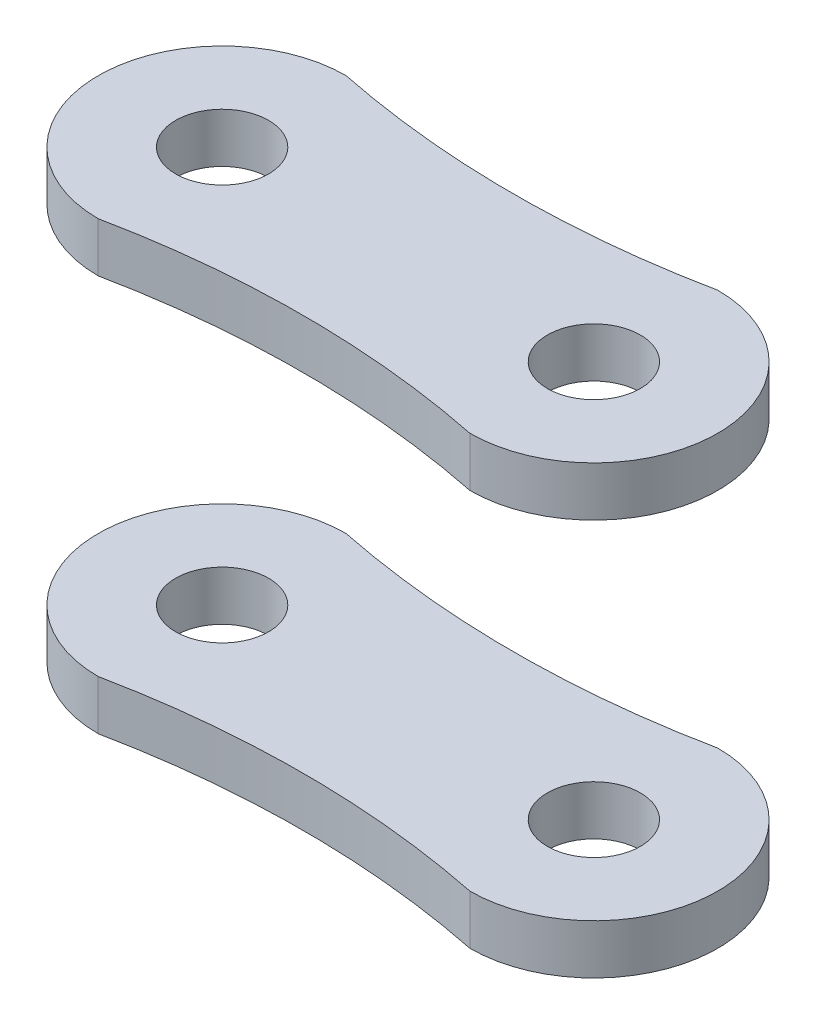
SolidWorks part; units mm, degrees
ref_plane "Front Plane" through (0, 0, 0) normal (0, 0, 1) x (1, 0, 0)
ref_plane "Top Plane" through (0, 0, 0) normal (0, 1, 0) x (1, 0, 0)
ref_plane "Right Plane" through (0, 0, 0) normal (1, 0, 0) x (0, 0, -1)
other "Configuration Table"
sketch "Sketch1" plane through (0, 0, 0) normal (0, 1, 0) x (1, 0, 0)
  line L0 (0, 0) -> (60, 0) construction
  arc A0 (0, 20) -> (0, -20) centre (0, 0) ccw
  arc A1 (60, -20) -> (60, 20) centre (60, 0) ccw
  arc A2 (0, 20) -> (60, 20) centre (30, 166.9694) ccw
  arc A3 (0, -20) -> (60, -20) centre (30, -166.9694) cw
  circle A4 centre (0, 0) radius 7.5
  circle A5 centre (60, 0) radius 7.5
  point P3 (30, 0)
  dimension "D2" = 20
  dimension "D3" = 15
  dimension "D4" = 15
  dimension "D1" = 60
extrude "Boss-Extrude1" add sketch "Sketch1" along normal blind 8
pattern_linear "LPattern1" count 2 spacing 64 along (0, 1, 0) of "Boss-Extrude1"
ref_plane "Plane1" through (0, 36, 0) normal (0, 1, 0) x (1, 0, 0)
sketch "Sketch5" plane through (0, 36, 0) normal (0, 1, 0) x (1, 0, 0)
  point P0 (0, 0)
sketch "Sketch6" plane through (0, 36, 0) normal (0, 1, 0) x (1, 0, 0)
  point P0 (60, 0)
